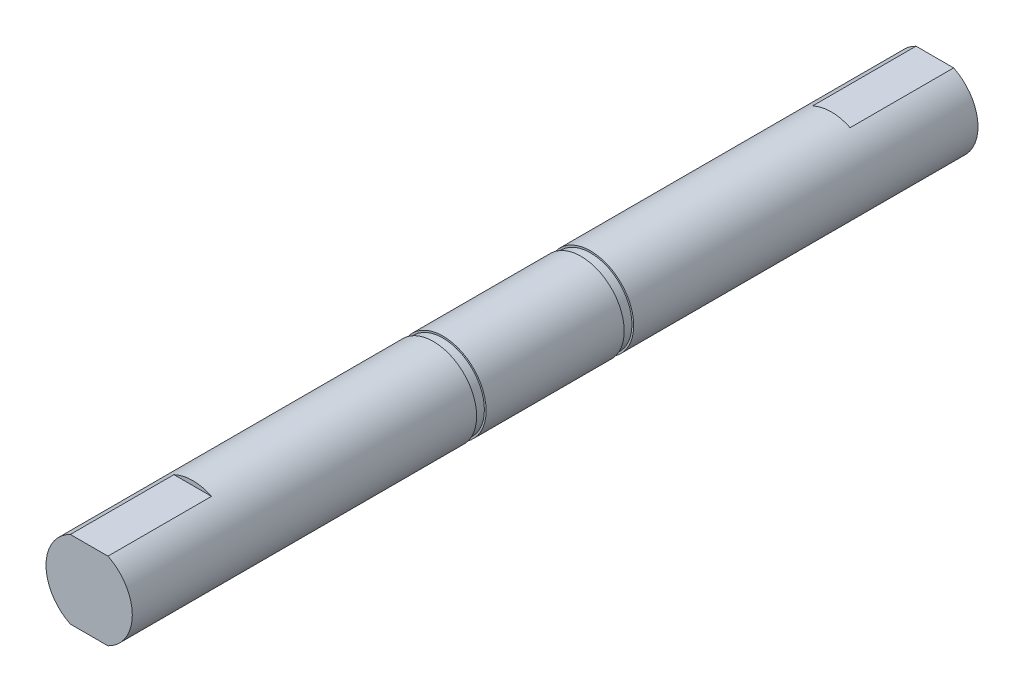
from build123d import *

# Parameters (mm, degrees)
SKETCH_1_R          = 5
EXTRUDE_1_DEPTH     = 49
CUT_EXTRUDE_START   = 1.1
SKETCH_3_R          = 5
SKETCH_3_R_2        = 4.8
CUT_EXTRUDE_2_DEPTH = 1.1
CUT_EXTRUDE_1_DEPTH = 12


with BuildPart() as part:
    # 草图1 → 凸台-拉伸1 (new, symmetric)
    with BuildSketch(Plane.XY):
        Circle(SKETCH_1_R)
    extrude(amount=EXTRUDE_1_DEPTH, both=True)

    # 草图3 → 切除-拉伸2 (cut)
    with BuildSketch(Plane.XY.offset(8).offset(CUT_EXTRUDE_START)):
        Circle(SKETCH_3_R)
        Circle(SKETCH_3_R_2, mode=Mode.SUBTRACT)
    cut_extrude_2 = extrude(amount=-CUT_EXTRUDE_2_DEPTH, mode=Mode.SUBTRACT)

    # 镜向2: 切除-拉伸2 across plane
    add(cut_extrude_2.mirror(Plane.XY), mode=Mode.SUBTRACT)

    # 草图2 → 切除-拉伸1 (cut)
    with BuildSketch(Plane.XY.offset(49)):
        with BuildLine():
            Line((-2.179449472, 4.5), (2.179449472, 4.5))
            ThreePointArc((2.179449472, 4.5), (0, 5), (-2.179449472, 4.5))
        make_face()
        with BuildLine():
            Line((-2.179449472, -4.5), (2.179449472, -4.5))
            ThreePointArc((2.179449472, -4.5), (0, -5), (-2.179449472, -4.5))
        make_face()
    cut_extrude_1 = extrude(amount=-CUT_EXTRUDE_1_DEPTH, mode=Mode.SUBTRACT)

    # 镜向1: 切除-拉伸1 across plane
    add(cut_extrude_1.mirror(Plane.XY), mode=Mode.SUBTRACT)


solid = part.part
